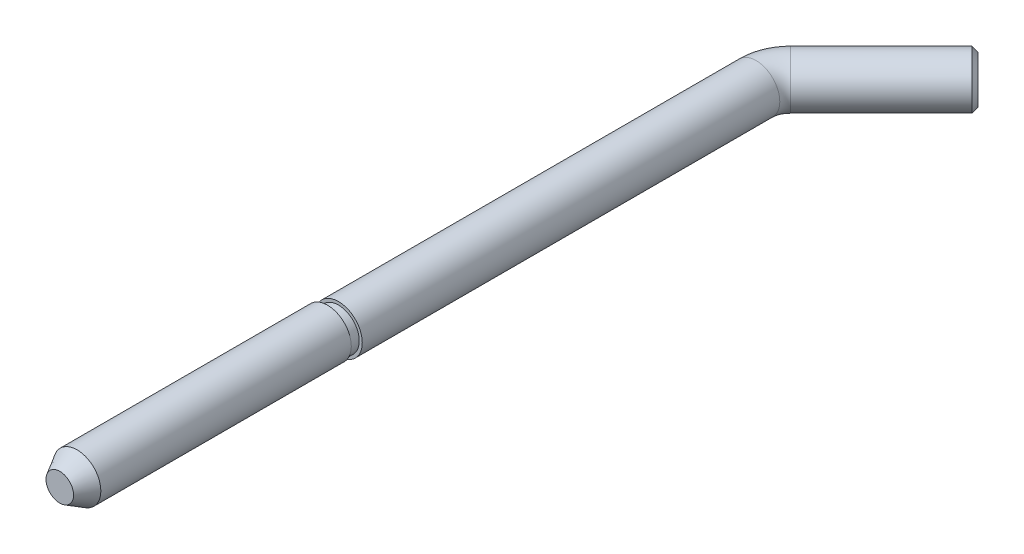
SolidWorks part; units mm, degrees
ref_plane "Front Plane" through (0, 0, 0) normal (0, 0, 1) x (1, 0, 0)
ref_plane "Top Plane" through (0, 0, 0) normal (0, 1, 0) x (1, 0, 0)
ref_plane "Right Plane" through (0, 0, 0) normal (1, 0, 0) x (0, 0, -1)
sketch "Sketch1" plane through (0, 0, 0) normal (0, 0, 1) x (1, 0, 0)
  circle A0 centre (0, 0) radius 2.75
  dimension "D1" = 5.5
sketch "Sketch2" plane through (0, 0, 0) normal (0, 1, 0) x (1, 0, 0)
  line L0 (0, 0) -> (0, 48.3431)
  line L1 (1.1716, 51.1716) -> (12.0208, 62.0208)
  arc A0 (0, 48.3431) -> (1.1716, 51.1716) centre (4, 48.3431) cw
  point P6 (0, 50)
  dimension "D4" = 4
  dimension "D1" = 50
  dimension "D2" = 17
  dimension "D3" = 135
sweep "Sweep1" add profiles "Sketch1" path "Sketch2"
sketch "Sketch4" plane through (0, 0, 0) normal (0, 0, 1) x (1, 0, 0)
  circle A0 centre (0, 0) radius 2.4
  dimension "D1" = 4.8
extrude "Boss-Extrude1" add sketch "Sketch4" along normal blind 1
sketch "Sketch5" plane through (0, 0, 1) normal (0, 0, 1) x (1, 0, 0)
  circle A0 centre (-0.2714, 0) radius 2.7531
extrude "Boss-Extrude2" add sketch "Sketch5" along normal blind 31
chamfer "Chamfer2" distance 2 angle 30 1 edges at (2.4817, 0, 32)
chamfer "Chamfer3" distance 0.5 angle 45 1 edges at (13.9654, 0, -60.0763)
